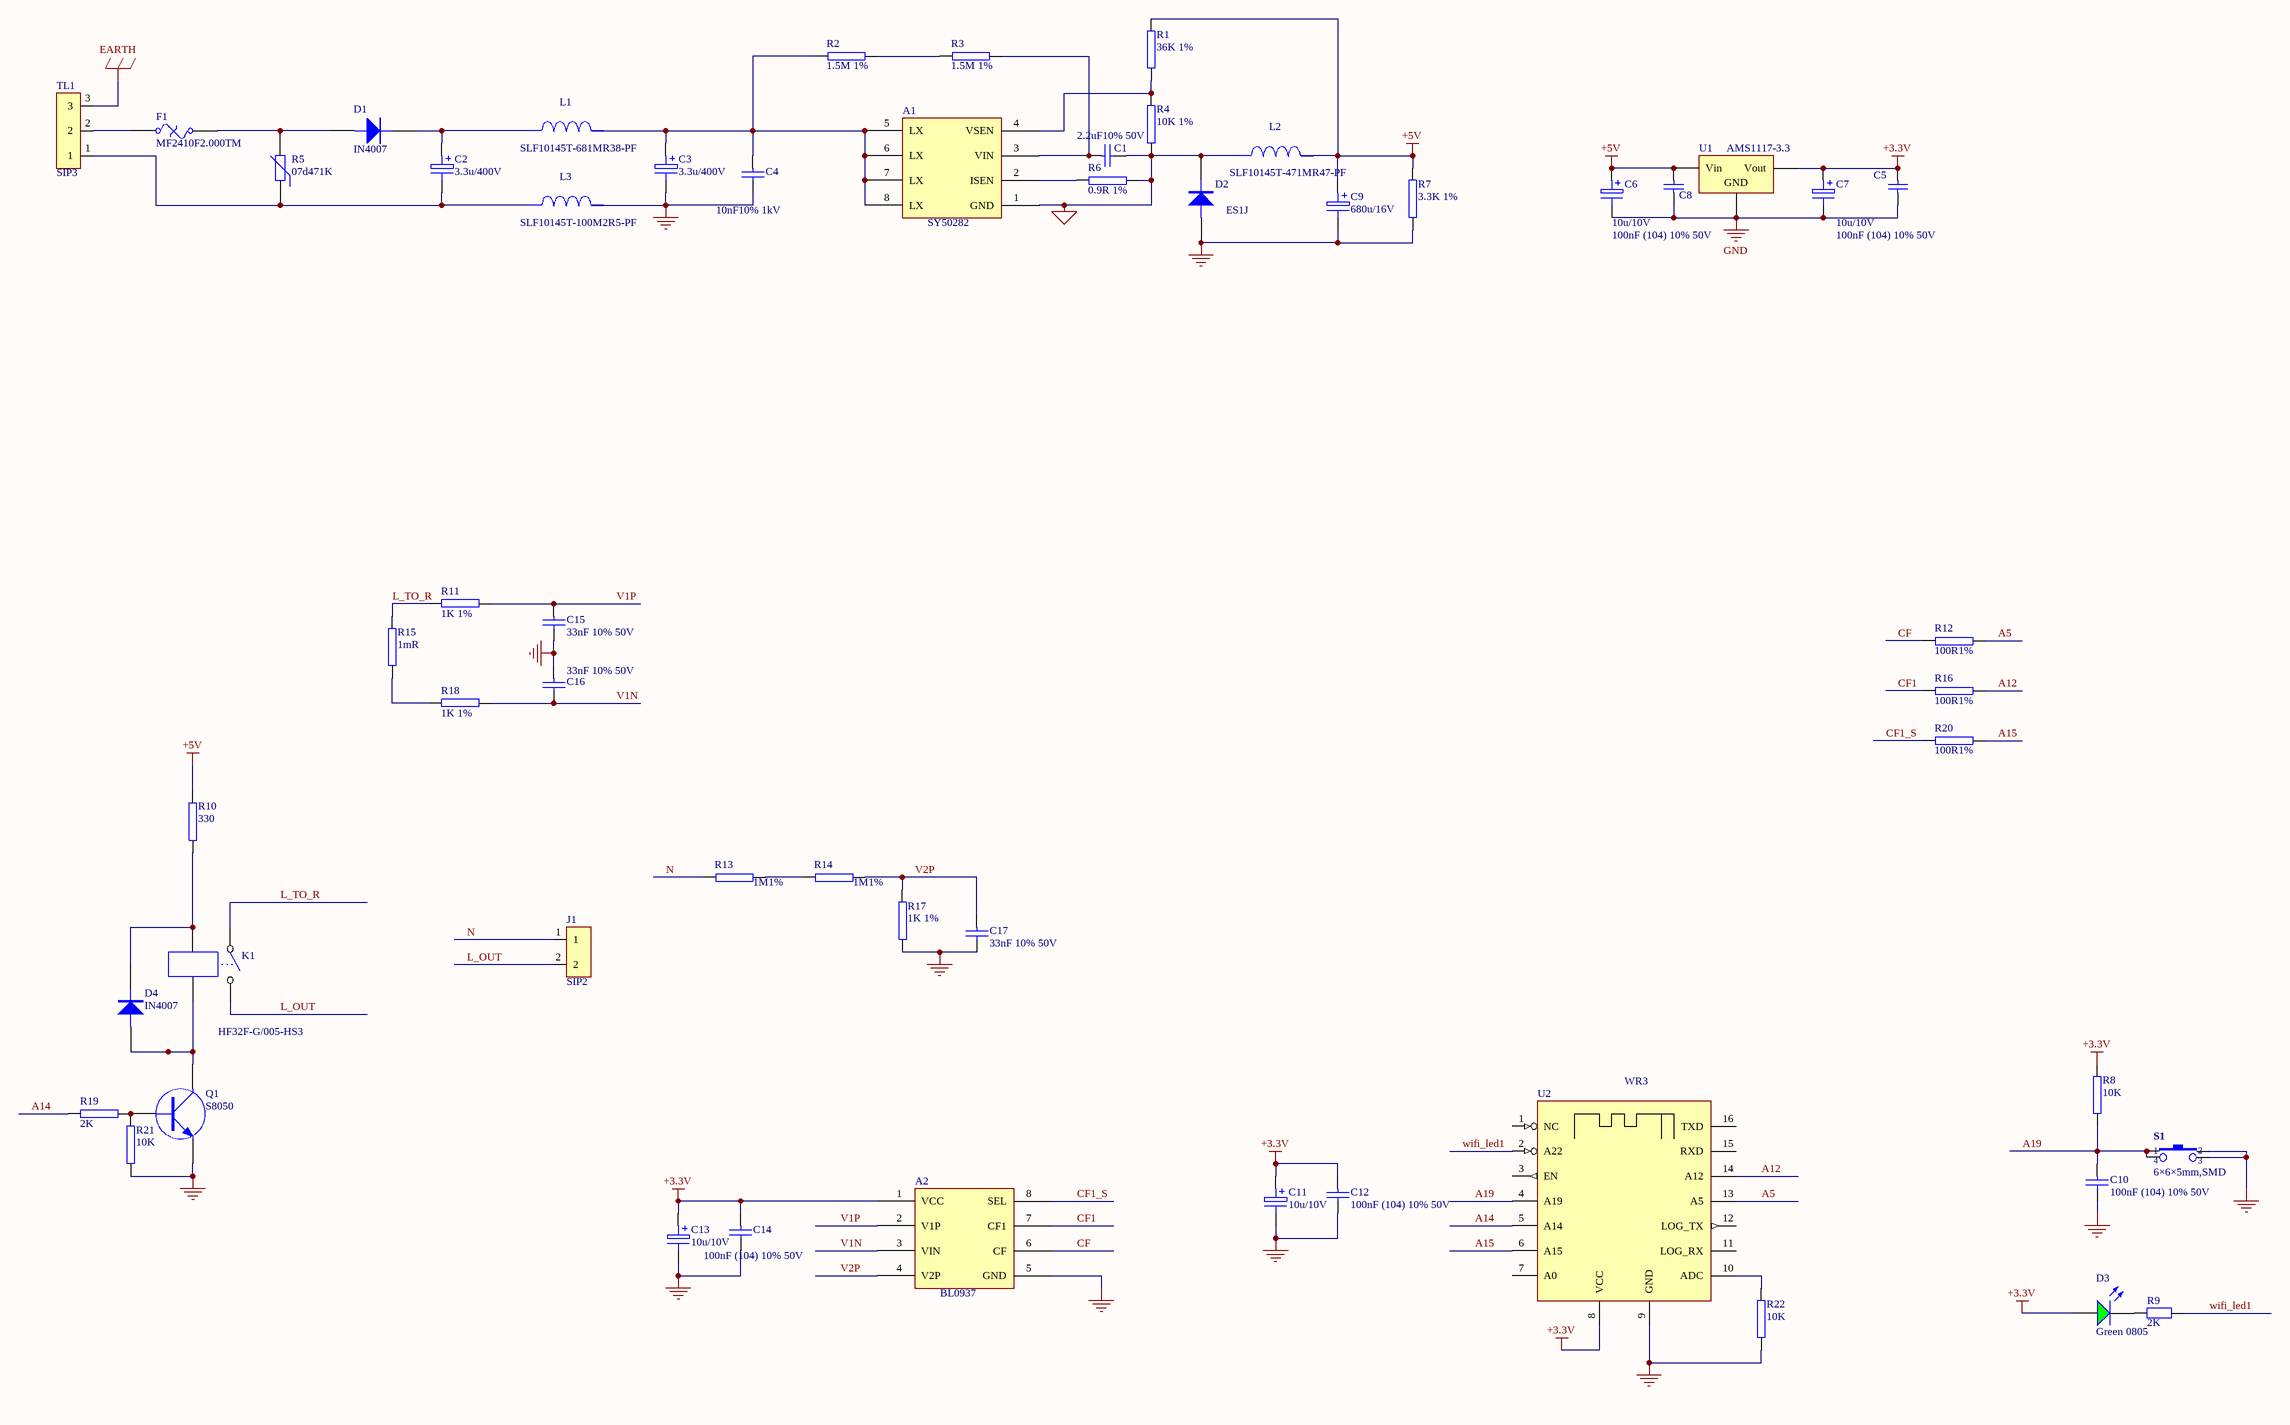
[diagram p0: MISC82282.SchDoc]
# Altium project MISC82282-3.PrjPCB
1 sheet, 56 parts. Net scope: global (net labels, ports and power ports of the same name join across sheets).
Board file: MISC82282.PcbDoc

## Sheet MISC82282.SchDoc
size A2

### Parts
A1  SY50282  [SO-8]
A2  BL0937  [SO-8]
C1  2.2uF10% 50V  [0603]
C2  3.3u/400V  [SMD8x10.5]
C3  3.3u/400V  [SMD8x10.5]
C4  10nF10% 1kV  [1206]
C5  100nF (104) 10% 50V  [0603]
C6  10u/10V  [0805]
C7  10u/10V  [0805]
C8  100nF (104) 10% 50V  [0603]
C9  680u/16V  [10X12.5]
C10  100nF (104) 10% 50V  [0603]
C11  10u/10V  [0805]
C12  100nF (104) 10% 50V  [0603]
C13  10u/10V  [0805]
C14  100nF (104) 10% 50V  [0603]
C15  33nF 10% 50V  [0603]
C16  33nF 10% 50V  [0603]
C17  33nF 10% 50V  [0603]
D1  IN4007  [SDIODE-2]
D2  ES1J  [SDIODE-2]
D3  Green 0805  [0805_LED_S1]
D4  IN4007  [SDIODE-2]
F1  MF2410F2.000TM  [2410]
J1  SIP2  [DIP-2]
K1  HF32F-G/005-HS3  [HF32F-G/005-HS3]
L1  value SLF10145T-681MR38-PF  [IND10X10]  (hidden comment: VLP8040T-3R3N)
L2  value SLF10145T-471MR47-PF  [IND10X10]  (hidden comment: VLP8040T-3R3N)
L3  value SLF10145T-100M2R5-PF  [IND10X10]  (hidden comment: VLP8040T-3R3N)
Q1  S8050  [SOT-23(SOT-23-3)]
R1  36K 1%  [1206]
R2  1.5M 1%  [1206]
R3  1.5M 1%  [1206]
R4  10K 1%  [0805]
R5  07d471K  [07d471K]
R6  0.9R 1%  [0805]
R7  3.3K 1%  [0805]
R8  10K  [0603]
R9  2K  [0603]
R10  330  [1206]
R11  1K 1%  [0603]
R12  100R1%  [0603]
R13  1M1%  [1206]
R14  1M1%  [1206]
R15  1mR  [2512]
R16  100R1%  [0603]
R17  1K 1%  [0603]
R18  1K 1%  [0603]
R19  2K  [0603]
R20  100R1%  [0603]
R21  10K  [0603]
R22  10K  [0603]
S1  value 6×6×5mm,SMD  [smd6X6x4.5]  (hidden comment: SW-PB4P)
TL1  SIP3  [DIP-3]
U1  AMS1117-3.3  [SOT-223]
U2  WR3  [WR3]

### Nets
+3.3V: A2.1(VCC) C5.1 C7.1 C11.1 C12.1 C13.1 C14.1 D3.A R8.1 U1.2(Vout) U2.8(VCC)
+5V: C6.1 C8.1 C9.1 L2.1 R1.1 R7.1 R10.2 U1.3(Vin)
EARTH: TL1.3
GND: A2.5(GND) C3.2 C4.2 C5.2 C6.2 C7.2 C8.2 C9.2 C10.2 C11.2 C12.2 C13.2 C14.2 C15.2 C16.1 C17.2 D2.A L3.1 Q1.2(E) R7.2 R17.2 R21.2 R22.2 S1.2 S1.3 U1.1(GND) U2.9(GND)
GNDS: A1.1(GND) C1.2 D2.K L2.2 R4.2 R6.2
A5: R12.2 U2.13(A5)
A12: R16.2 U2.14(A12)
A14: R19.2 U2.5(A14)
A15: R20.2 U2.6(A15)
A19: C10.1 R8.2 S1.1 S1.4 U2.4(A19)
CF: A2.6(CF) R12.1
CF1: A2.7(CF1) R16.1
CF1_S: A2.8(SEL) R20.1
L_OUT: J1.2 K1.4
L_TO_R: K1.3 R11.2 R15.1
N: J1.1 R13.1
V1N: A2.3(VIN) C16.2 R18.1
V1P: A2.2(V1P) C15.1 R11.1
V2P: A2.4(V2P) C17.1 R14.2 R17.1
wifi_led1: R9.1 U2.2(A22)
NetA1_2: A1.2(ISEN) R6.1
NetA1_3: A1.3(VIN) C1.1 R3.2
NetA1_4: A1.4(VSEN) R1.2 R4.1
NetA1_5: A1.5(LX) A1.6(LX) A1.7(LX) A1.8(LX) C3.1 C4.1 L1.1 R2.1
NetC2_1: C2.1 D1.K L1.2
NetC2_2: C2.2 L3.2 R5.1 TL1.1
NetD1_A: D1.A F1.2 R5.2
NetD3_K: D3.K R9.2
NetD4_A: D4.A K1.2 Q1.3(C)
NetD4_K: D4.K K1.1 R10.1
NetF1_1: F1.1 TL1.2
NetQ1_1: Q1.1(B) R19.1 R21.1
NetR2_2: R2.2 R3.1
NetR13_2: R13.2 R14.1
NetR15_2: R15.2 R18.2
NetR22_1: R22.1 U2.10(ADC)

Not connected (* = marked no-connect by the designer): U2 1(NC) 3(EN) 7(A0) 11(LOG_RX) 12(LOG_TX) 15(RXD) 16(TXD)

### Library data of the parts
A1 A2 = TPS54331DR
C1 C4 C10 C12 C14-C17 = CAP: Capacitor
C2 C3 C6 C7 C9 C11 C13 = ELECTRO1
C5 C8 = 0603 100nF (104) 10% 50V: SMD capacitor; ComponentLink1Description: Supplier link; ComponentLink1URL: http://www.szlcsc.com/product/details_15331.html; Package: 0603; Supplier: LC; SuppliersPartNumber: C14663
D1 D2 D4 = DIODE
D3 = 0805 翠绿: LED; ComponentLink1Description: Supplier link; ComponentLink1URL: http://www.szlcsc.com/product/details_2670.html; Package: 0805; Supplier: LC; SuppliersPartNumber: C2297
F1 = Fuse Thermal: Thermal Fuse; Published: 24-Mar-1999; LatestRevisionDate: 17-Jul-2002; LatestRevisionNote: Re-released for DXP Platform.; PackageReference: PIN-W2/E2.8; Publisher: Altium Limited
K1 = RELAY-SPST
L1-L3 = VLP8040T-3R3N: Unknown; Manufacturer Name: TDK; PackageReference: VLP8040T-3R3N; Manufacturer Part Number: VLP8040T-3R3N
Q1 = NPN-1
R1-R4 R6-R8 R10-R22 = RES2
R5 = Res Varistor: Varistor (Voltage-Sensitive Resistor); Published: 24-Mar-1999; LatestRevisionDate: 29-May-2009; LatestRevisionNote: IPC-7351 Footprint Added.; PackageVersion: Mar-2003; PackageReference: 6-0805; PackageDescription: Chip Resistor 0805 Case Size; Code_IPC: RESC2012; Publisher: Altium Limited
R9 = 0603 680Ω (6800) 1%: SMD resistor; ComponentLink1Description: Supplier link; ComponentLink1URL: http://www.szlcsc.com/product/details_23955.html; Package: 0603; Supplier: LC; SuppliersPartNumber: C23228
S1 = SW-PB4P: 6×6×5.0mm, black, SMD,,*; 物料代码: 1.09.01.0003; 名称: Tact switch; 贴片和直插: SMT; 型号: 6×6×5.0mm, black, SMD; ComponentLink1Description: ErpDataInfo
U1 = SOT-223 AMS1117-3.3: Low-dropout linear regulator (LDO); ComponentLink1Description: Supplier link; ComponentLink1URL: http://www.szlcsc.com/product/details_6652.html; Package: SOT-223; Supplier: LC; SuppliersPartNumber: C6186
U2 = SR_FRS_1WV